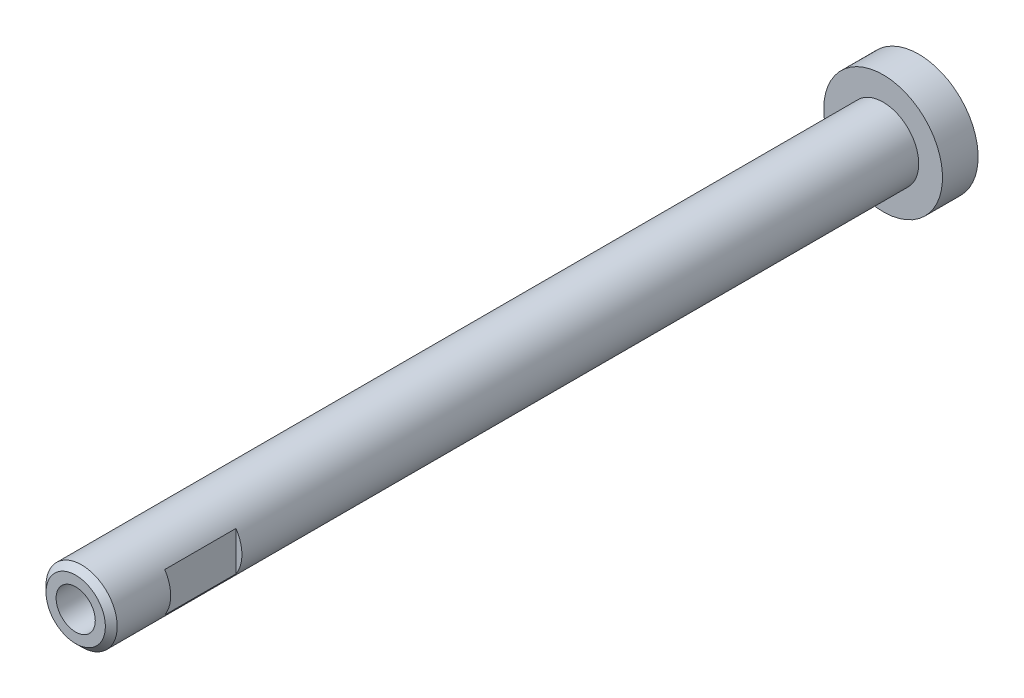
SolidWorks part; units mm, degrees
material "Cr12"
ref_plane "前视基准面" through (0, 0, 0) normal (0, 0, 1) x (1, 0, 0)
ref_plane "上视基准面" through (0, 0, 0) normal (0, 1, 0) x (1, 0, 0)
ref_plane "右视基准面" through (0, 0, 0) normal (1, 0, 0) x (0, 0, -1)
sketch "草图1" plane through (0, 0, 0) normal (0, 0, 1) x (1, 0, 0)
  circle A0 centre (0, 0) radius 3
  dimension "D1" = 6
extrude "凸台-拉伸1" add sketch "草图1" along normal blind 71
hole_wizard "M4 螺纹孔2" positions "草图6" profile "草图5" tap size "M4" standard "GB"
sketch "草图6" plane through (0, 0, 71) normal (0, 0, 1) x (1, 0, 0)
  point P0 (0, 0)
sketch "草图5" plane through (0, 0, 71) normal (1, 0, 0) x (0, -1, 0)
  line L0 (0, 0) -> (0, 12.4914)
  line L1 (0, 12.4914) -> (1.65, 11.5)
  line L2 (1.65, 11.5) -> (1.65, 0)
  line L5 (1.65, 0) -> (0, 0)
  line L10 (0, 12.4914) -> (-1.65, 11.5) construction
  line L11 (0, -6.35) -> (0, 107.95) construction
  dimension "螺纹孔钻头直径" = 3.3
  dimension "螺纹孔钻头深度" = 11.5
  dimension "导头角度" = 118
cosmetic thread "孔螺蚊线3" parameters "D1"=8, "D2"=4
chamfer "倒角1" distance 0.5 angle 45 1 edges at (3, 0, 71)
sketch "Sketch1" plane through (0, 0, 0) normal (0, 1, 0) x (1, 0, 0)
  line L0 (-2.5, -63) -> (2.5, -63) construction
  line L1 (-5.1971, -60) -> (-2.5, -60)
  line L2 (-5.1971, -60) -> (-5.1971, -66)
  line L3 (-5.1971, -66) -> (-2.5, -66)
  line L4 (-2.5, -60) -> (-2.5, -66)
  line L5 (4.8618, -60) -> (2.5, -60)
  line L6 (4.8618, -60) -> (4.8618, -66)
  line L7 (4.8618, -66) -> (2.5, -66)
  line L8 (2.5, -60) -> (2.5, -66)
  line L9 (0, -71) -> (0, -63) construction
  line L10 (-2.5, -71) -> (2.5, -71) construction
  dimension "D1" = 6
  dimension "D2" = 5
  dimension "D3" = 5
extrude "Extrude1" cut sketch "Sketch1" against normal through all and the other way through all
sketch "Sketch4" plane through (0, 0, 0) normal (0, 0, -1) x (-1, 0, 0)
  circle A0 centre (0, 0) radius 5
  circle A1 centre (0, 0) radius 3
  circle A2 centre (0, 0) radius 3 construction
  dimension "D1" = 10
extrude "Extrude2" add sketch "Sketch4" against normal blind 3
